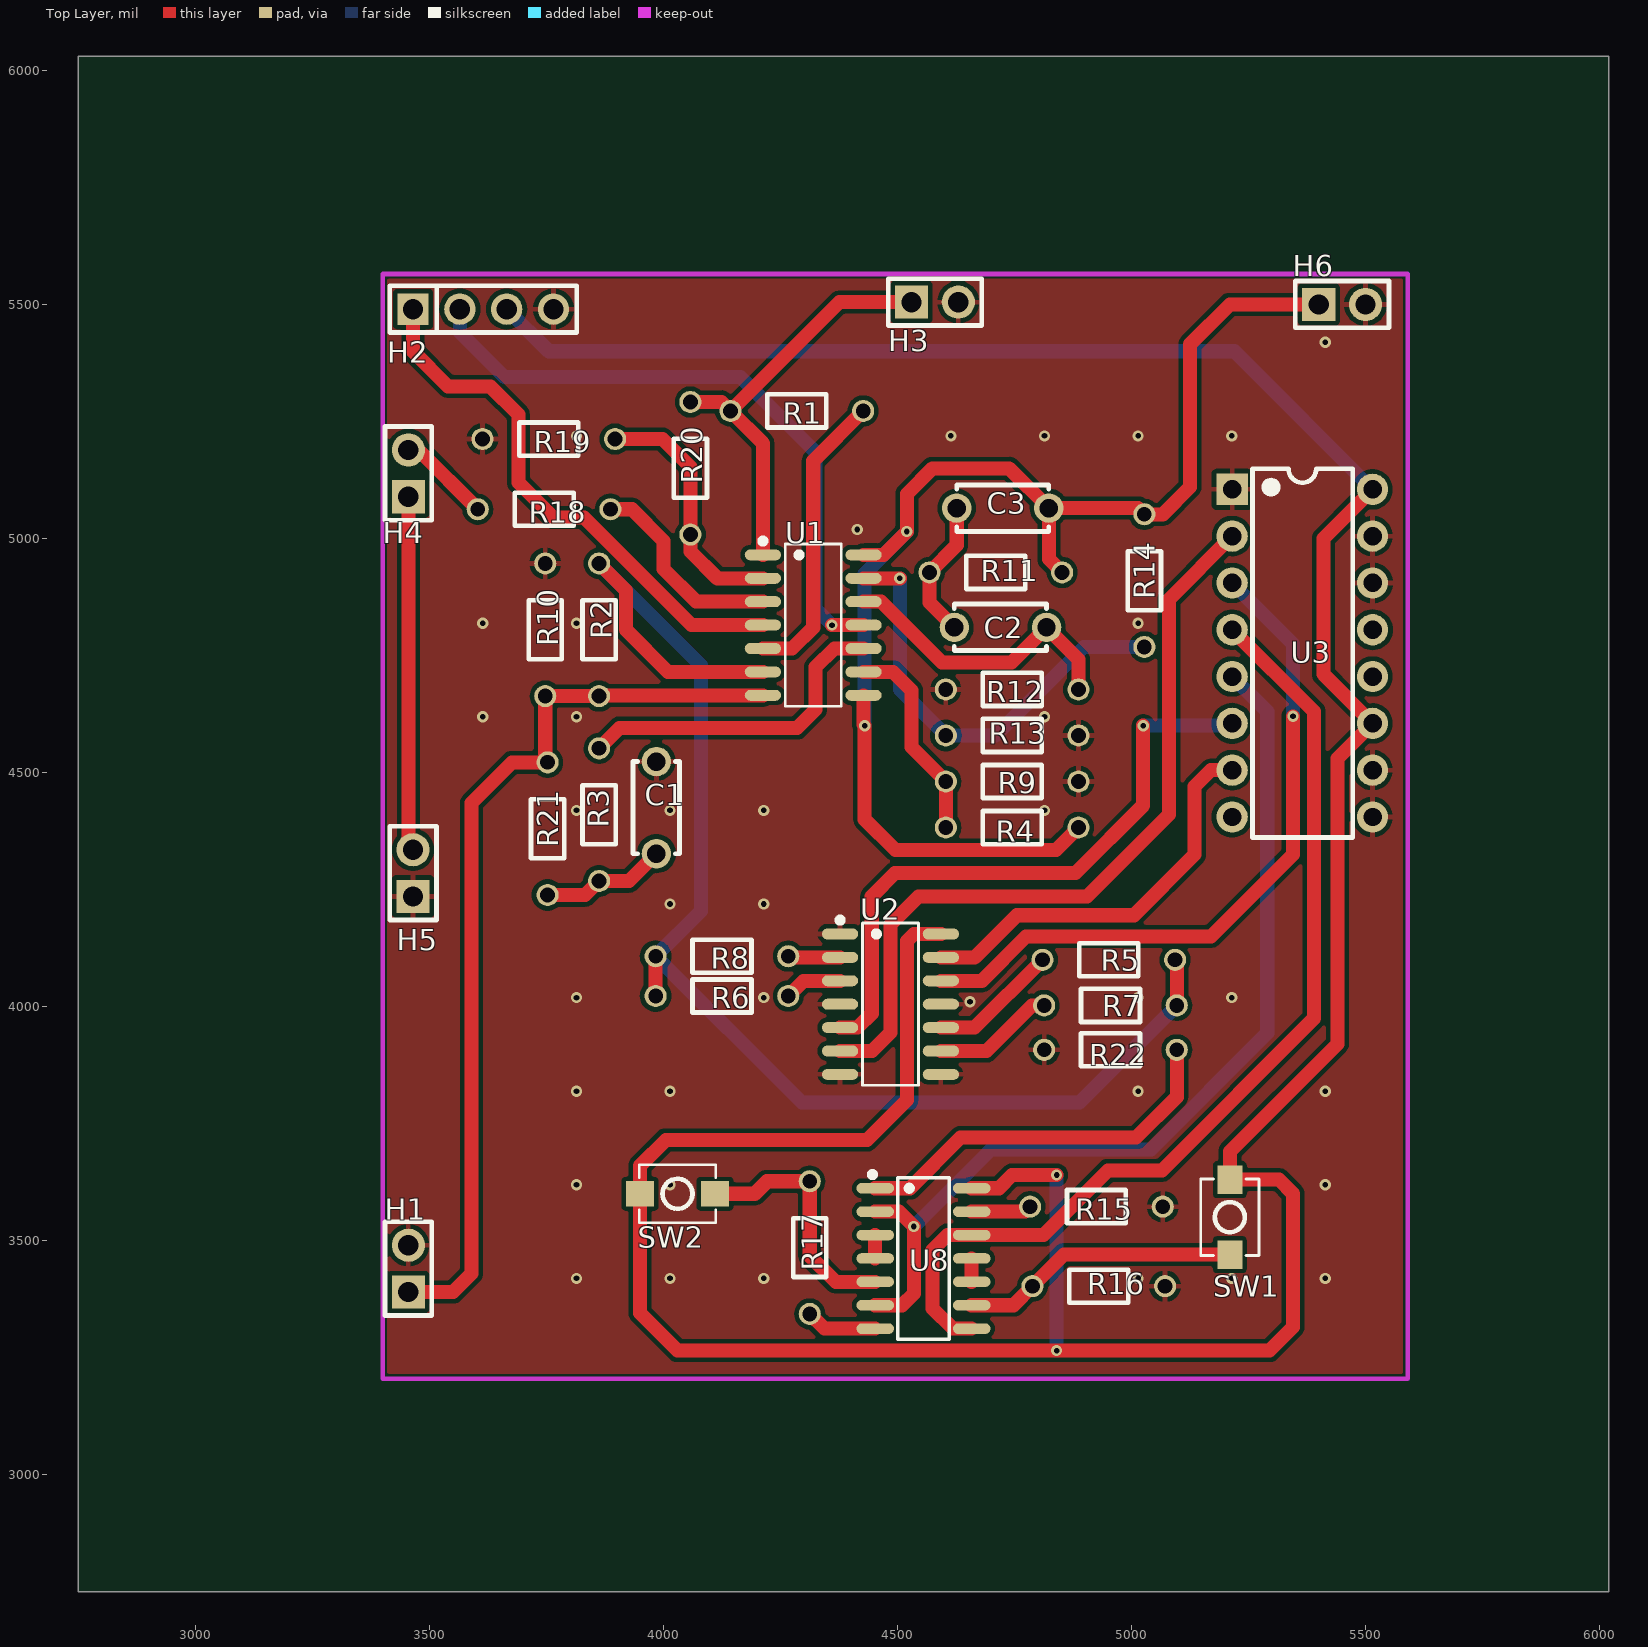
[diagram p0: Top Layer view]
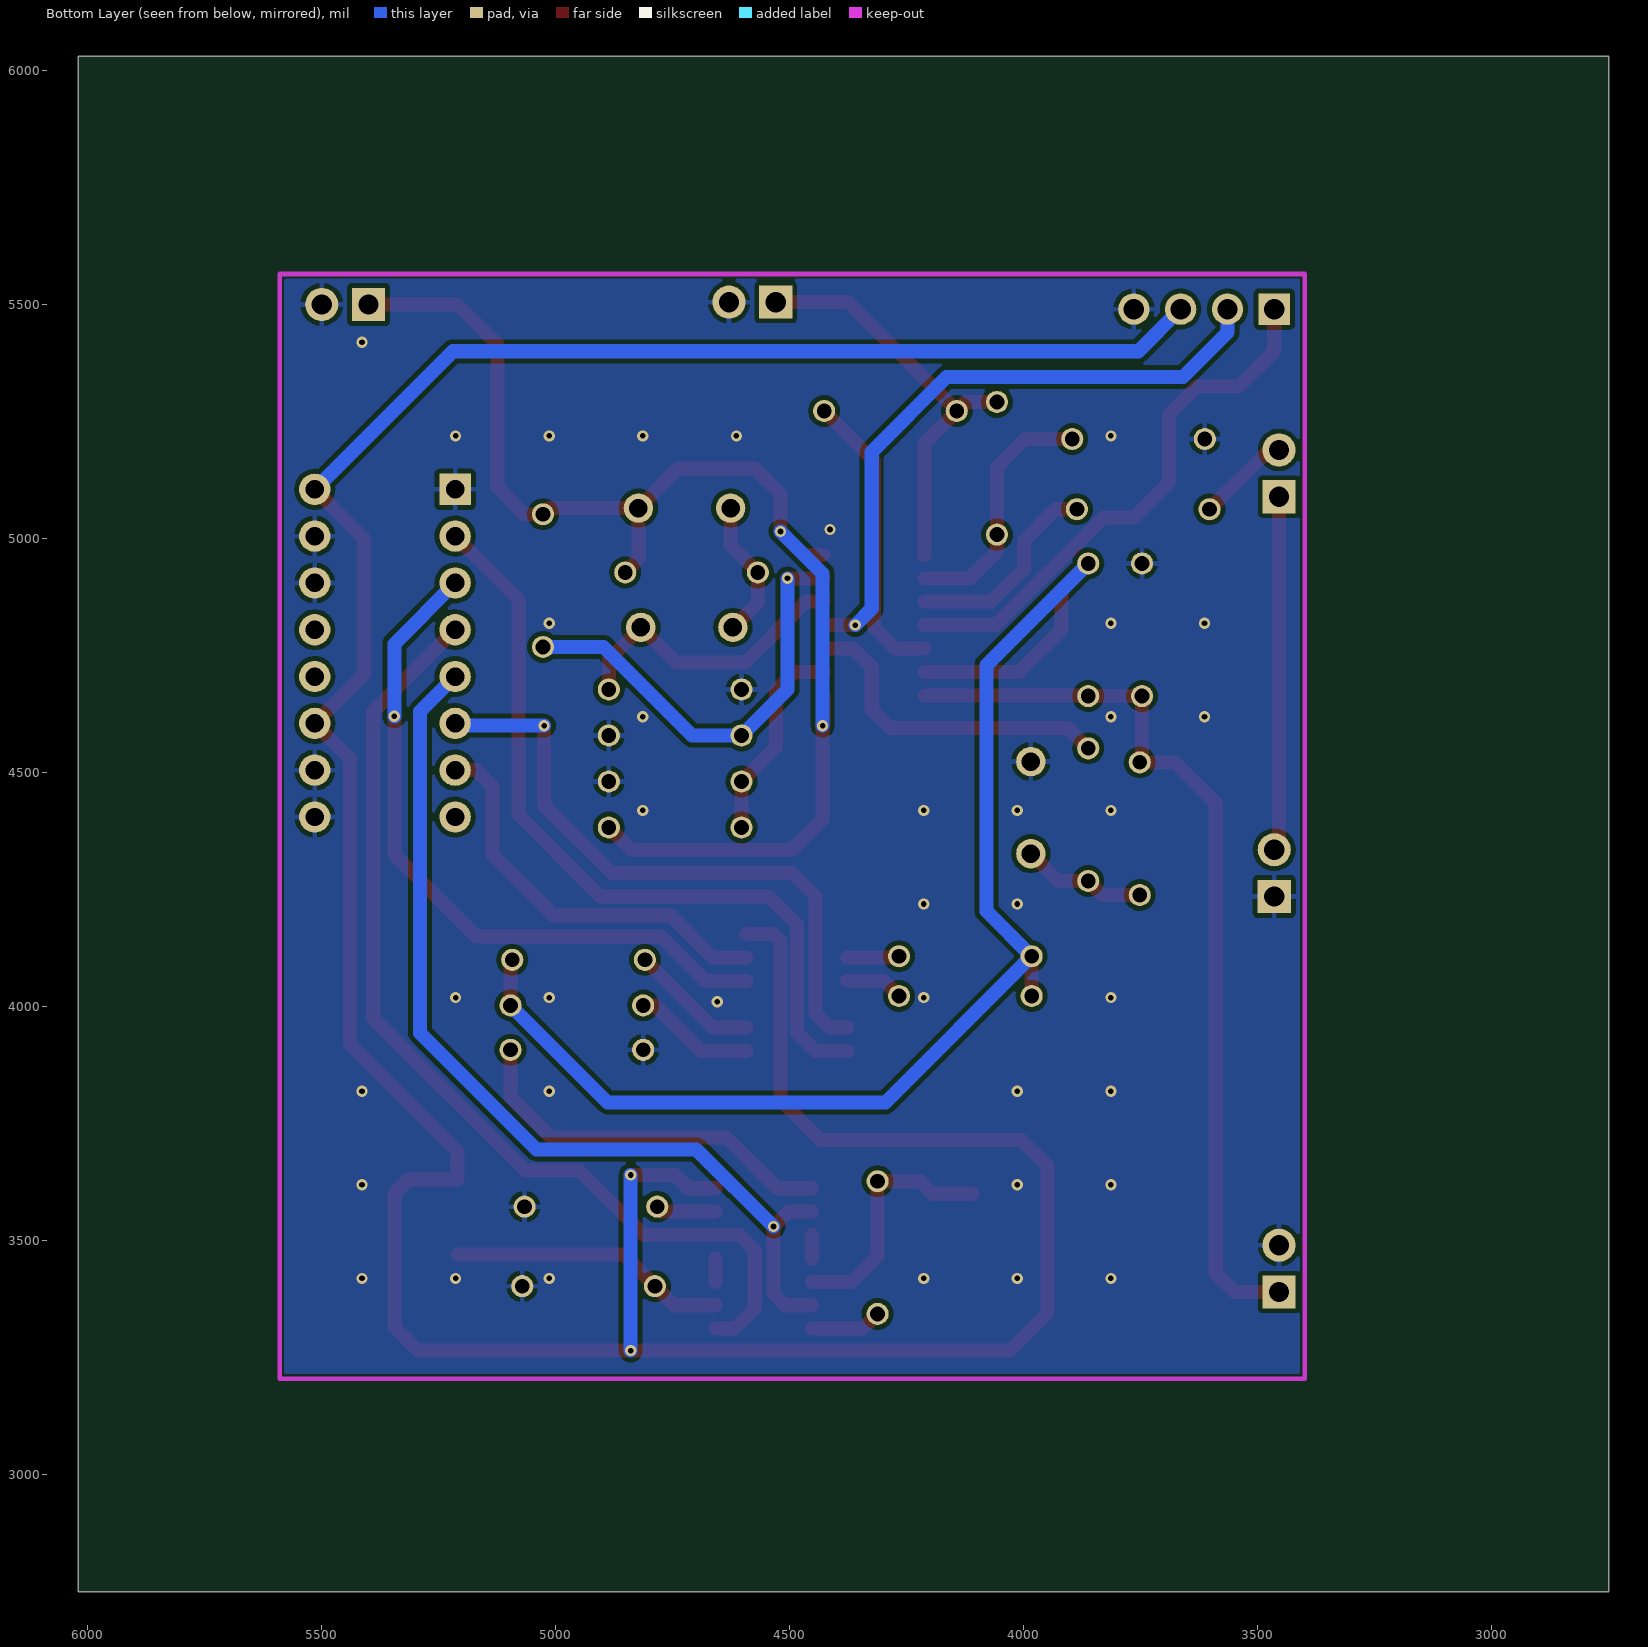
[diagram p1: Bottom Layer view, seen from below]
# Altium PCB MISC51958.pcbdoc
Units mil, origin at the board's own origin, x right, y up, seen from the top; angles counter-clockwise.
Board outline 3270 x 3280 mil, 2 copper layers (Top Layer, Bottom Layer), stack 62.206 mil thick; 37 components, 36 nets, 126 pads, 46 vias.

## Layer stack, top to bottom
Top Solder Mask Layer: solder mask 0.394, Dk 3.3
Top Layer: signal copper 1.379
Dielectric1: surface 59.449, FR4, Dk 4.5
Bottom Layer: signal copper 1.378
Bottom Solder Mask Layer: solder mask 0.394, Dk 3.3

## Board outline
6020,2750 2750,2750 2750,6030 6020,6030

## Design rules (kind name [scope] priority, off if disabled: settings)
BoardOutlineClearance copperThickness2oz_1 [All] p2 off: genericclearance=7.99 ignorepadtopadclearanceinfootprint=FALSE except(0: Arc-SplitContinuation Track-SplitContinuation SMDPad-SplitContinuation THPad-SplitContinuation Via-SplitContinuation Fill-SplitContinuation Region-SplitContinuation Poly-SplitContinuation Text-SplitContinuation Hole-SplitContinuation; 5.98: Arc-CutoutEdge SMDPad-CutoutEdge THPad-CutoutEdge Via-CutoutEdge Fill-CutoutEdge Region-CutoutEdge Text-CutoutEdge; 6.93: Hole-OutlineEdge Hole-CutoutEdge; 10: Poly-OutlineEdge Poly-CutoutEdge; 11.81: Arc-OutlineEdge Track-OutlineEdge SMDPad-OutlineEdge THPad-OutlineEdge Via-OutlineEdge Fill-OutlineEdge Region-OutlineEdge Text-OutlineEdge Track-CutoutEdge)
BoardOutlineClearance copperThickness1oz_1 [All] p4: genericclearance=4.02 ignorepadtopadclearanceinfootprint=FALSE except(0: Arc-SplitContinuation Track-SplitContinuation SMDPad-SplitContinuation THPad-SplitContinuation Via-SplitContinuation Fill-SplitContinuation Region-SplitContinuation Poly-SplitContinuation Text-SplitContinuation Hole-SplitContinuation; 6: SMDPad-CutoutEdge THPad-CutoutEdge Via-CutoutEdge Fill-CutoutEdge Region-CutoutEdge Text-CutoutEdge; 6.93: Hole-OutlineEdge Hole-CutoutEdge; 10: Poly-OutlineEdge Poly-CutoutEdge; 11.8: Arc-OutlineEdge Track-OutlineEdge SMDPad-OutlineEdge THPad-OutlineEdge Via-OutlineEdge Fill-OutlineEdge Region-OutlineEdge Text-OutlineEdge; 11.81: Arc-CutoutEdge Track-CutoutEdge)
Clearance copperThickness2oz [All] p1 off: gap=7.99 ignorepadtopadclearanceinfootprint=FALSE except(5.98: SMDPad-Track SMDPad-SMDPad THPad-Track SMDPad-THPad THPad-THPad Track-Via SMDPad-Via THPad-Via Via-Via Fill-Track Region-Track Fill-SMDPad Region-SMDPad Fill-THPad Region-THPad Fill-Via Region-Via Fill-Fill Fill-Region Region-Region Arc-Track Arc-SMDPad Arc-THPad Arc-Via Fill-Arc Region-Arc Arc-Arc Text-Track SMDPad-Text Text-THPad Text-Via Fill-Text Region-Text Arc-Text Text-Text; 6.93: Hole-Track Hole-SMDPad Hole-THPad Hole-Via Fill-Hole Region-Hole Hole-Arc Hole-Text; 10: Poly-Track Poly-SMDPad Poly-THPad Poly-Via Poly-Fill Poly-Region Poly-Poly Poly-Arc Poly-Text Poly-Hole)
Clearance copperThickness1oz [All] p3: gap=4.02 ignorepadtopadclearanceinfootprint=FALSE except(5.98: SMDPad-Track SMDPad-SMDPad THPad-Track SMDPad-THPad THPad-THPad Track-Via SMDPad-Via THPad-Via Via-Via Fill-Track Region-Track Fill-SMDPad Region-SMDPad Fill-THPad Region-THPad Fill-Via Region-Via Fill-Fill Fill-Region Region-Region; 6: Arc-Track Arc-SMDPad Arc-THPad Arc-Via Fill-Arc Region-Arc Arc-Arc Text-Track SMDPad-Text Text-THPad Text-Via Fill-Text Region-Text Arc-Text Text-Text; 6.93: Hole-Track Hole-SMDPad Hole-THPad Hole-Via Fill-Hole Region-Hole Hole-Arc Hole-Text; 10: Poly-Track Poly-SMDPad Poly-THPad Poly-Via Poly-Fill Poly-Region Poly-Poly Poly-Arc Poly-Text Poly-Hole)
DiffPairsRouting differentialPair [All] p1: maxlimit=6 minlimit=6 mostfreqgap=6 toplayer_minwidth=5 toplayer_prefwidth=10 toplayer_maxwidth=100 toplayer_mingap=6 toplayer_prefgap=6 toplayer_maxgap=6 bottomlayer_minwidth=5 bottomlayer_prefwidth=10 bottomlayer_maxwidth=100 bottomlayer_mingap=6 bottomlayer_prefgap=6 bottomlayer_maxgap=6 maxuncoupledlength=10
HoleToHoleClearance otherClearance [All] p1: gap=11.81 allowstackedmicrovias=TRUE
Length netLength [All] p1: minlimit=0 maxlimit=0
MatchedLengths netLengthTolerance [All] p1: tolerance=1000
PasteMaskExpansion pasteMaskExpansion [All] p1: expansion=0
PlaneConnect innerPlane [All] p1: planeconnectstyle=Relief reliefexpansion=20 reliefentries=4 reliefconductorwidth=10 reliefairgap=10
PolygonConnect copperRegion [(InNet('GND'))] p1: connectstyle=Relief reliefconductorwidth=10 reliefentries=4 polygonreliefangle="90 Angle" airgapwidth=10 via.connectstyle=Relief via.reliefconductorwidth=10 via.reliefentries=4 via.polygonreliefangle="90 Angle" via.airgapwidth=10
RoutingVias viaSize [All] p1: holewidth=12.01 width=24.02 viastyle="Through Hole" minholewidth=11.81 minwidth=19.68 maxholewidth=248.03 maxwidth=393.7
SolderMaskExpansion solderMaskExpansion [IsVia] p1: expansion=-1000 istentingtop=TRUE
SolderMaskExpansion solderMaskExpansion [All] p2: expansion=2 istentingtop=FALSE
Width copperThickness2oz_2 [All] p1 off: maxlimit=100 minlimit=8 preferedwidth=10
Width copperThickness1oz_2 [All] p2: maxlimit=100 minlimit=5 preferedwidth=10

## Components (designator, comment, footprint, x,y, rotation, side; value= is the part's Value field where it differs from the comment)
C1 "10nF" CAP-TH_L5.0-W2.5-P5.00-D1.0 3985,4425 r270 top
C2 "100nF" CAP-TH_L5.0-W2.5-P5.00-D1.0 4720,4810 r180 top
C3 "100nF" CAP-TH_L5.0-W2.5-P5.00-D1.0 4725,5065 r0 top
H1 "" HDR-TH_2P-P2.54-V-M-1 3455,3440 r90 top
H2 "" HDR-TH_4P-P2.54-V-M 3615,5490 r0 top
H3 "" HDR-TH_2P-P2.54-V-M-1 4580,5505 r0 top
H4 "" HDR-TH_2P-P2.54-V-M-1 3455,5139.14 r90 top
H5 "" HDR-TH_2P-P2.54-V-M-1 3465,4285 r90 top
H6 "" HDR-TH_2P-P2.54-V-M-1 5450,5500 r0 top
R1 "15K" Res_1/8W 4285,5270 r0 top
R2 "1200K" Res_1/8W 3860,4805 r270 top
R3 "47K" Res_1/8W 3865,4410 r90 top
R4 "120K" Res_1/8W 4745,4380 r0 top
R5 "80K" Res_1/8W 4951.39,4097.32 r0 top
R6 "40K" Res_1/8W 4125,4025 r180 top
R7 "20K" Res_1/8W 4955,4000 r0 top
R8 "10K" Res_1/8W 4125,4110 r180 top
R9 "230K" Res_1/8W 4745,4483.29 r180 top
R10 "80K" Res_1/8W 3745,4805 r270 top
R11 "15K" Res_1/8W 4710,4925 r0 top
R12 "15K" Res_1/8W 4745,4675 r0 top
R13 "80K" Res_1/8W 4745,4581.62 r180 top
R14 "51K" Res_1/8W 5025,4910 r270 top
R15 "15K" Res_1/8W 4925,3570 r0 top
R16 "15K" Res_1/8W 4930,3405 r180 top
R17 "1K" Res_1/8W 4315,3485 r90 top
R18 "10K" Res_1/8W 3745,5060 r0 top
R19 "10K" Res_1/8W 3755,5210 r0 top
R20 "90K" Res_1/8W 4060,5150 r90 top
R21 "120K" Res_1/8W 3750,4380 r270 top
R22 "15K" Res_1/8W 4955,3910 r180 top
SW1 "" Key_SMD_3x4x2 5210,3550 r90 top
SW2 "" Key_SMD_3x4x2 4030,3600 r180 top
U1 "LM324ADR" SOP-14_L8.6-W3.9-P1.27-LS6.0-BL 4320,4815 r270 top
U2 "CD4066BD" SOP-14_L8.6-W3.9-P1.27-LS6.0-BL 4485,4005 r270 top
U3 "NTE74193" PDIP-16_L19.7-W6.6-P2.54-LS7.6-BL 5365,4755 r270 top
U8 "SN74LS00DR" SOIC-14_L8.7-W3.9-P1.27-LS6.0-BL 4555.44,3461.82 r270 top

## Footprints (in the part's own frame and the unit in brackets; to place one, negate y for a bottom-side part, rotate by r counter-clockwise, add the part's x,y. Pads: shape width x height; smd on the part's side, far side on the other; paste and mask are expansions set on the pad)
CAP-TH_L5.0-W2.5-P5.00-D1.0 [mm]
  round 1.6 hole 1: 1(-2.5,0) 2(2.5,0)
  silkscreen extent -2.5,-1.27 2.5,1.25
HDR-TH_2P-P2.54-V-M-1 [mm]
  rect 1.8x1.8 hole 1.1: 1(-1.27,0)
  round 1.8 hole 1.1: 2(1.27,0)
  silkscreen extent -2.54,-1.27 2.54,1.27
HDR-TH_4P-P2.54-V-M [mm]
  rect 1.7x1.7 hole 1.1: 1(-3.81,0)
  round 1.7 hole 1.1: 2(-1.27,0) 3(1.27,0) 4(3.81,0)
  silkscreen extent -5.08,-1.27 5.08,1.27
Key_SMD_3x4x2 [mm]
  rect 1.53x1.36 smd paste+0 mask+0.051: 1(-2.035,0) 2(2.035,0)
  silkscreen extent -2.08,-1.58 2.08,1.58
PDIP-16_L19.7-W6.6-P2.54-LS7.6-BL [mm]
  rect 1.7x1.7 hole 1: 1(-8.89,-3.81)
  round 1.7 hole 1: 2(-6.35,-3.81) 3(-3.81,-3.81) 4(-1.27,-3.81) 5(1.27,-3.81) 6(3.81,-3.81) 7(6.35,-3.81) 8(8.89,-3.81) 9(8.89,3.81) 10(6.35,3.81) 11(3.81,3.81) 12(1.27,3.81) 13(-1.27,3.81) 14(-3.81,3.81) 15(-6.35,3.81) 16(-8.89,3.81)
  silkscreen extent -10,-2.7 10,2.73
Res_1/8W [mil]
  round 47.2 hole 31.5 paste+0 mask+2: 1(-141.7,2.48) 2(141.7,2.48)
  silkscreen extent -63,-33 63,38
SOIC-14_L8.7-W3.9-P1.27-LS6.0-BL [mil]
  oval 22.6x80.24 smd: 1(-150,-103.11) 2(-100,-103.11) 3(-50,-103.11) 4(0,-103.11) 5(50,-103.11) 6(100,-103.11) 7(150,-103.11) 8(150,103.11) 9(100,103.11) 10(50,103.11) 11(0,103.11) 12(-50,103.11) 13(-100,103.11) 14(-150,103.11)
  silkscreen extent -185,-115 172,55
SOP-14_L8.6-W3.9-P1.27-LS6.0-BL [mm]
  oval 0.595x1.968 smd: 1(-3.81,-2.734) 2(-2.54,-2.734) 3(-1.27,-2.734) 4(0,-2.734) 5(1.27,-2.734) 6(2.54,-2.734) 7(3.81,-2.734) 8(3.81,2.734) 9(2.54,2.734) 10(1.27,2.734) 11(0,2.734) 12(-1.27,2.734) 13(-2.54,2.734) 14(-3.81,2.734)
  silkscreen extent -4.71,-2.88 4.4,1.52

## Via types
v1: diameter 24.02, hole 12, Top Layer to Bottom Layer, 46 vias

## Nets (pads, with @x,y where several pads share a name; then routed paths per layer and width w, separated by ;. In a path a pad name is that pad's centre, name@x,y a point inside that pad or via, vN(x,y) a via of type N, cw(c..) or ccw(c..) an arc to the next point about the centre after c; other vN are vias at no path point)
5V: H2.3 SW1.2 SW2.2 U2.14 U3.11 U3.16 U8.14 | length 7509.1
  Top Layer w30: U2.14 4535,4155 4520,4140 4520,3800 4435,3715 4005,3715 3949.88,3659.88 SW2.2 3949.88,3345.12 4030,3265 v1(4840,3265) 5295,3265 5345,3315 5345,3600 5314.88,3630.12 SW1.2 5210,3690 5440,3920 5440,4530 U3.11 5410,4710 5410,5000 U3.16 ; U8.14 4716.82,3611.82 4745,3640 v1(4840,3640)
  Bottom Layer w30: H2.3 3755,5400 5220,5400 U3.16 ; v1(4840,3265) v1(4840,3640)
12V: H2.1 U1.4 | length 1164.6
  Top Layer w30: H2.1 3465,5400 3540,5325 3630,5325 3690,5265 3690,5120 3765,5045 3830,5045 4060,4815 U1.4
$1N60: R18.2 U1.3 | length 442.6
  Top Layer w30: R18.2 3932.52,5062.48 4000,4995 4000,4935 4070,4865 U1.3
$1N64: H4.2 R18.1 | length 200.8
  Top Layer w30: H4.2 3476.64,5189.14 R18.1
$1N65: H4.1 H5.2 | length 758.3
  Top Layer w30: H4.1 3455,4345 H5.2
$1N69: H3.1 R1.1 R20.2 U1.1 | length 912.8
  Top Layer w30: R20.2 4124.08,5291.7 R1.1 ; U1.1 4212.37,5203.41 R1.1 ; H3.1 4375.82,5505 R1.1
$1N70: R19.2 R20.1 U1.2 | length 544.3
  Top Layer w30: R19.2 3997.52,5212.48 4057.52,5152.48 R20.1 4057.52,4972.48 4115,4915 U1.2
$1N71: R1.2 U1.5 | length 632.9
  Top Layer w30: U1.5 4275,4765 4320,4810 4320,5165.78 R1.2
$1N74: R8.1 U2.2 | length 111.7
  Top Layer w30: R8.1 4269.22,4105 U2.2
$1N76: U3.5 U8.2 U8.6 | length 2051
  Top Layer w30: U8.6 4510,3361.82 4535,3386.82 v1(4535,3530) 4503.18,3561.82 U8.2
  Bottom Layer w30: v1(4535,3530) 4700,3695 5041.63,3695 5290,3943.37 5290,4630 U3.5
$1N77: U3.4 U8.8 U8.12 | length 2149
  Top Layer w30: U8.8 4618.18,3311.82 4575,3355 4575,3480 4606.82,3511.82 U8.12 4811.82,3511.82 4950,3650 5065,3650 5390,3975 5390,4630 U3.4
$1N81: U2.13 U3.7 | length 873
  Top Layer w30: U2.13 4665,4105 4755,4195 5005,4195 5135,4325 5135,4470 5170,4505 U3.7
$1N82: U2.5 U3.6 | length 1352.9
  Top Layer w30: U2.5 4415,3955 4445,3985 4445,4235 4495,4285 4880,4285 5025,4430 v1(5025,4600)
  Bottom Layer w30: v1(5025,4600) 5210,4600 U3.6
$1N83: U2.6 U3.2 | length 1697.8
  Top Layer w30: U2.6 4445.58,3905 4485,3944.42 4485,4175 4545,4235 4905,4235 5080,4410 5080,4870 U3.2
$1N84: U2.12 U3.3 | length 1498.1
  Top Layer w30: U2.12 4680,4055 4775,4150 5170,4150 5345,4325 v1(5345,4620)
  Bottom Layer w30: U3.3 5345,4775 v1(5345,4620)
$1N86: R7.1 U2.9 | length 261
  Top Layer w30: U2.9 4690,3905 4787.48,4002.48 R7.1
$1N87: R6.1 U2.3 | length 124.1
  Top Layer w30: R6.1 4299.18,4055 U2.3
$1N88: R5.1 U2.10 | length 277
  Top Layer w30: U2.10 4664.9,3955 R5.1
$1N90: R2.1 R5.2 R6.2 R7.2 R8.2 U1.6 | length 2977.1
  Top Layer w30: R2.1 3920,4889.18 3920,4805 4010,4715 U1.6 ; R6.2 R8.2 ; R5.2 5096.7,4096.19 R7.2
  Bottom Layer w30: R2.1 4080,4729.18 4080,4204.22 R8.2 4295.82,3795 4889.22,3795 R7.2
$1N92: R3.2 U1.10 | length 706.2
  Top Layer w30: R3.2 3905.82,4595 4285,4595 4325,4635 4325,4725 4365,4765 U1.10
$1N93: C1.2 R3.1 R21.2 | length 269.1
  Top Layer w30: R21.2 3832.52,4238.3 R3.1 3926.72,4268.3 C1.2
$1N94: R4.1 R9.2 U1.9 | length 441.8
  Top Layer w30: U1.9 4490,4715 4530,4675 4530,4554.11 R9.2 R4.1
$1N97: H1.1 R2.2 R10.2 R21.1 U1.7 | length 1964.2
  Top Layer w30: H1.1 3550,3390 3590,3430 3590,4435 3676.7,4521.7 R21.1 3747.48,4526.7 R10.2 R2.2 3864.18,4665 U1.7
$1N98: C2.1 R12.2 U1.12 | length 636.5
  Top Layer w30: U1.12 4465,4865 4595,4735 4743.43,4735 C2.1 4886.7,4741.73 R12.2
$1N99: C2.2 C3.1 R11.1 | length 301.2
  Top Layer w30: C2.2 4568.3,4863.27 R11.1 4626.57,4985.75 C3.1
$1N103: R13.2 R14.2 U1.13 | length 956.5
  Top Layer w30: U1.13 v1(4505,4915)
  Bottom Layer w30: v1(4505,4915) 4505,4677.44 R13.2 4709.14,4579.14 4898.3,4768.3 R14.2
$1N104: C3.2 H6.1 R4.2 R11.2 R14.1 U1.8 U1.14 | length 2872.5
  Top Layer w30: U1.8 4427.63,4602.37 v1(4430,4600) 4430,4400 4495.98,4334.02 4838.24,4334.02 R4.2 ; U1.14 4470,4965 v1(4520,5015) 4520,5095 4575,5150 4738.43,5150 C3.2 ; R11.2 4823.43,4955.75 C3.2 ; H6.1 5210,5500 5125,5415 5125,5110 5066.7,5051.7 R14.1 5014.18,5065 C3.2
  Bottom Layer w30: v1(4430,4600) 4430,4925 v1(4520,5015)
$1N106: R15.1 U8.13 | length 129.2
  Top Layer w30: U8.13 4772.64,3561.82 R15.1
$1N109: U8.10 U8.11 | length 50
  Top Layer w30: U8.10 U8.11
$1N110: R16.2 SW1.1 U8.9 | length 596.2
  Top Layer w30: U8.9 4747.59,3361.82 R16.2 4855.66,3469.88 SW1.1
$1N113: U8.3 U8.4 | length 50
  Top Layer w30: U8.4 U8.3
$1N114: R17.2 SW2.1 U8.5 | length 535.5
  Top Layer w30: SW2.1 4195,3600 4221.7,3626.7 R17.2 4312.52,3467.48 4368.18,3411.82 U8.5
$1N116: R17.1 U8.7 | length 152.8
  Top Layer w30: R17.1 4344.01,3311.82 U8.7
$1N118: R22.1 U8.1 | length 825.9
  Top Layer w30: U8.1 4526.82,3611.82 4635,3720 5010,3720 5096.7,3806.7 R22.1
-12V: H2.2 U1.11 | length 1367.8
  Top Layer w30: v1(4360,4815) U1.11
  Bottom Layer w30: H2.2 3565,5440 3660,5345 4165,5345 4325,5185 4325,4850 v1(4360,4815)
GND: C1.1 H1.2 H2.4 H3.2 H5.1 H6.2 R9.1 R10.1 R12.1 R13.1 R15.2 R16.1 R19.1 R22.2 U2.1 U2.4 U2.7 U2.8 U2.11 U3.1 U3.9 U3.10 U3.14 U3.15
  other v1: 3814.1,3419.1 4014.1,3419.1 4214.1,3419.1 5014.1,3419.1 5214.1,3419.1 5414.1,3419.1 3814.1,3619.1 4014.1,3619.1 5414.1,3619.1 3814.1,3819.1 4014.1,3819.1 5014.1,3819.1 5414.1,3819.1 4655,4010 3814.1,4019.1 4214.1,4019.1 5014.1,4019.1 5214.1,4019.1 4014.1,4219.1 4214.1,4219.1 3814.1,4419.1 4014.1,4419.1 4214.1,4419.1 4814.1,4419.1 3614.1,4619.1 3814.1,4619.1 4814.1,4619.1 3614.1,4819.1 3814.1,4819.1 5014.1,4819.1 4414.1,5019.1 3814.1,5219.1 4614.1,5219.1 4814.1,5219.1 5014.1,5219.1 5214.1,5219.1 5414.1,5419.1
pads on no net: U3.8 U3.12 U3.13

## Polygon pours and split planes (outlines as drawn)
GND on Top Layer (solid, remove dead copper, pour order 0): 3000,5780 3000,3000 5770,3000 5770,5780
GND on Bottom Layer (solid, remove dead copper, pour order 2): 3235,5765 3235,3130 5750,3130 5750,5765

## Keep-outs
Board Outline Layer:
  lines w10: 3400,3205 3400,5565 5590,5565 5590,3205 3400,3205